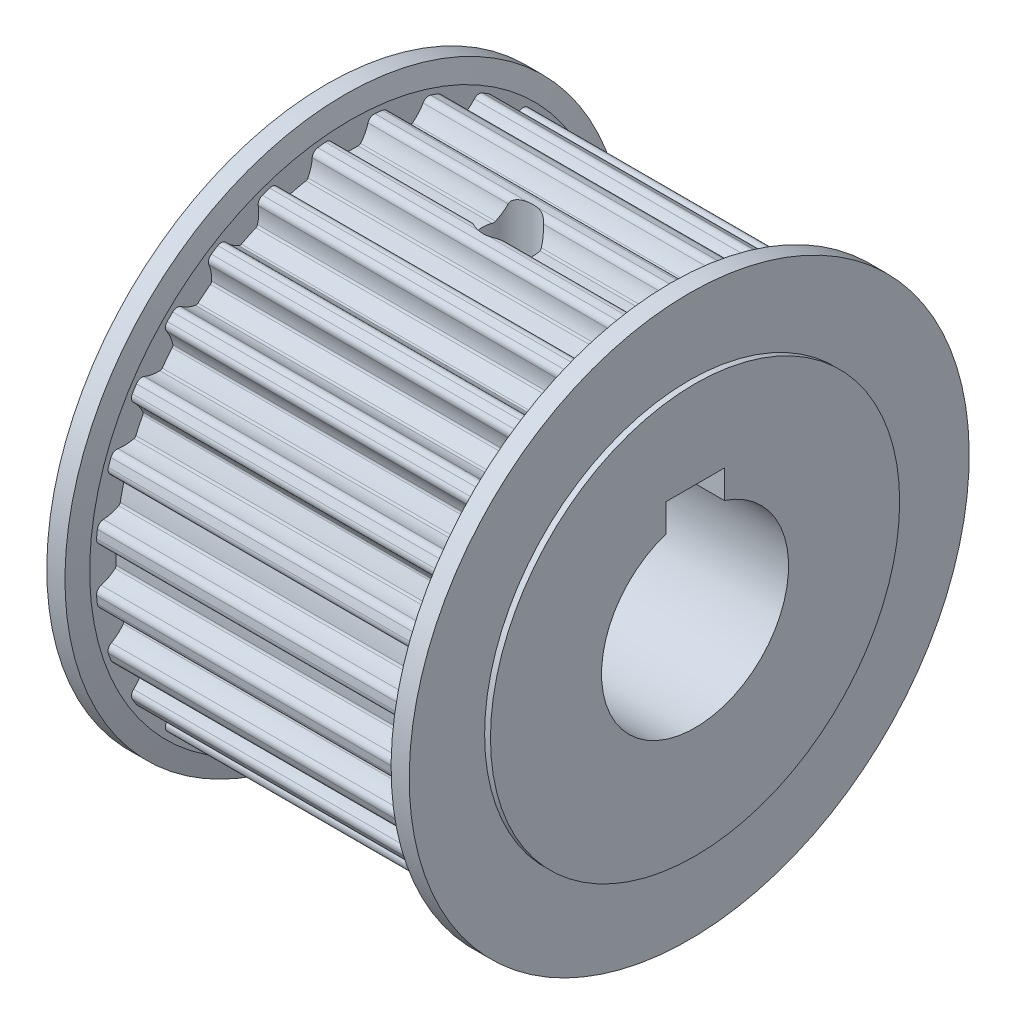
from build123d import *

# Parameters (mm, degrees)
CUT_EXTRUDE1_DEPTH       = 43.67001289
FILLET1_R                = 0.25
FILLET2_R                = 0.55
CIRPATTERN1_COUNT        = 28
FILLET1_OF_CIRPATTERN1_R = 0.25
FILLET2_OF_CIRPATTERN1_R = 0.55
CUT_EXTRUDE4_DEPTH       = 47.596190831
SKETCH24_W               = 2.15
SKETCH24_H               = 21.8
SKETCH25_W               = 2.15
SKETCH25_H               = 21.8


with BuildPart() as part:
    # Sketch1 → Revolve1 (revolve)
    with BuildSketch(Plane.XY, mode=Mode.PRIVATE) as revolve1_sk:
        Polygon((-13.5, 21.8), (-13.5, 17.5), (-16, 17.5), (-16, 0), (16, 0), (16, 17.5), (13.5, 17.5), (13.5, 21.8), align=None)
    revolve(revolve1_sk.sketch.rotate(Axis((16, 0, 0), (-1, 0, 0)), 90), axis=Axis((16, 0, 0), (-1, 0, 0)))

    # Sketch2 → Cut-Extrude1 (cut, through all)
    with BuildSketch(Plane(origin=(13.5, 0, 0), x_dir=(0, 0, -1), z_dir=(1, 0, 0))):
        with BuildLine():
            ThreePointArc((1.625, 21.739350841), (0, 21.8), (-1.625, 21.739350841))
            ThreePointArc((-1.625, 21.739350841), (-1.343515659, 20.815447254), (-0.804781532, 20.013825888))
            ThreePointArc((-0.804781532, 20.013825888), (0, 20.03), (0.804781532, 20.013825888))
            ThreePointArc((0.804781532, 20.013825888), (1.343515659, 20.815447254), (1.625, 21.739350841))
        make_face()
    cut_extrude1 = extrude(amount=-CUT_EXTRUDE1_DEPTH, mode=Mode.SUBTRACT)

    # Fillet1
    fillet1_edges = [part.edges().sort_by_distance(p)[0] for p in [
        (0, 20.013825888, -0.804781532),
        (0, 20.013825888, 0.804781532),
    ]]
    fillet(fillet1_edges, radius=FILLET1_R)

    # Fillet2
    fillet2_edges = [part.edges().sort_by_distance(p)[0] for p in [
        (0, 21.739350841, -1.625),
        (0, 21.739350841, 1.625),
    ]]
    fillet(fillet2_edges, radius=FILLET2_R)

    # CirPattern1: Cut-Extrude1 ×28 about axis
    cirpattern1_axis = Axis((0, 0, 0), (1, 0, 0))
    for i in range(1, CIRPATTERN1_COUNT):
        add(cut_extrude1.rotate(cirpattern1_axis, i * 360 / CIRPATTERN1_COUNT), mode=Mode.SUBTRACT)

    # Fillet1 of CirPattern1
    fillet1_of_cirpattern1_edges = [part.edges().sort_by_distance(p)[0] for p in [
        (0, 19.691118226, 3.66889125),
        (0, 19.33295675, 5.238099208),
        (0, 18.381015673, 7.958590504),
        (0, 17.682652433, 9.408756716),
        (0, 16.149212242, 11.849212799),
        (0, 15.145666086, 13.107619876),
        (0, 13.107619876, 15.145666086),
        (0, 11.849212799, 16.149212242),
        (0, 9.408756716, 17.682652433),
        (0, 7.958590504, 18.381015673),
        (0, 5.238099208, 19.33295675),
        (0, 3.66889125, 19.691118226),
        (0, 0.804781532, 20.013825888),
        (0, -0.804781532, 20.013825888),
        (0, -3.66889125, 19.691118226),
        (0, -5.238099208, 19.33295675),
        (0, -7.958590504, 18.381015673),
        (0, -9.408756716, 17.682652433),
        (0, -11.849212799, 16.149212242),
        (0, -13.107619876, 15.145666086),
        (0, -15.145666086, 13.107619876),
        (0, -16.149212242, 11.849212799),
        (0, -17.682652433, 9.408756716),
        (0, -18.381015673, 7.958590504),
        (0, -19.33295675, 5.238099208),
        (0, -19.691118226, 3.66889125),
        (0, -20.013825888, 0.804781532),
        (0, -20.013825888, -0.804781532),
        (0, -19.691118226, -3.66889125),
        (0, -19.33295675, -5.238099208),
        (0, -18.381015673, -7.958590504),
        (0, -17.682652433, -9.408756716),
        (0, -16.149212242, -11.849212799),
        (0, -15.145666086, -13.107619876),
        (0, -13.107619876, -15.145666086),
        (0, -11.849212799, -16.149212242),
        (0, -9.408756716, -17.682652433),
        (0, -7.958590504, -18.381015673),
        (0, -5.238099208, -19.33295675),
        (0, -3.66889125, -19.691118226),
        (0, -0.804781532, -20.013825888),
        (0, 0.804781532, -20.013825888),
        (0, 3.66889125, -19.691118226),
        (0, 5.238099208, -19.33295675),
        (0, 7.958590504, -18.381015673),
        (0, 9.408756716, -17.682652433),
        (0, 11.849212799, -16.149212242),
        (0, 13.107619876, -15.145666086),
        (0, 15.145666086, -13.107619876),
        (0, 16.149212242, -11.849212799),
        (0, 17.682652433, -9.408756716),
        (0, 18.381015673, -7.958590504),
        (0, 19.33295675, -5.238099208),
        (0, 19.691118226, -3.66889125),
    ]]
    fillet(fillet1_of_cirpattern1_edges, radius=FILLET1_OF_CIRPATTERN1_R)

    # Fillet2 of CirPattern1
    fillet2_of_cirpattern1_edges = [part.edges().sort_by_distance(p)[0] for p in [
        (0, 21.555896446, 3.253202796),
        (0, 20.83270341, 6.42171851),
        (0, 20.291539392, 7.968276419),
        (0, 18.88141724, 10.896425239),
        (0, 18.009679824, 12.28378739),
        (0, 15.983337968, 14.824739708),
        (0, 14.824739708, 15.983337968),
        (0, 12.28378739, 18.009679824),
        (0, 10.896425239, 18.88141724),
        (0, 7.968276419, 20.291539392),
        (0, 6.42171851, 20.83270341),
        (0, 3.253202796, 21.555896446),
        (0, 1.625, 21.739350841),
        (0, -1.625, 21.739350841),
        (0, -3.253202796, 21.555896446),
        (0, -6.42171851, 20.83270341),
        (0, -7.968276419, 20.291539392),
        (0, -10.896425239, 18.88141724),
        (0, -12.28378739, 18.009679824),
        (0, -14.824739708, 15.983337968),
        (0, -15.983337968, 14.824739708),
        (0, -18.009679824, 12.28378739),
        (0, -18.88141724, 10.896425239),
        (0, -20.291539392, 7.968276419),
        (0, -20.83270341, 6.42171851),
        (0, -21.555896446, 3.253202796),
        (0, -21.739350841, 1.625),
        (0, -21.739350841, -1.625),
        (0, -21.555896446, -3.253202796),
        (0, -20.83270341, -6.42171851),
        (0, -20.291539392, -7.968276419),
        (0, -18.88141724, -10.896425239),
        (0, -18.009679824, -12.28378739),
        (0, -15.983337968, -14.824739708),
        (0, -14.824739708, -15.983337968),
        (0, -12.28378739, -18.009679824),
        (0, -10.896425239, -18.88141724),
        (0, -7.968276419, -20.291539392),
        (0, -6.42171851, -20.83270341),
        (0, -3.253202796, -21.555896446),
        (0, -1.625, -21.739350841),
        (0, 1.625, -21.739350841),
        (0, 3.253202796, -21.555896446),
        (0, 6.42171851, -20.83270341),
        (0, 7.968276419, -20.291539392),
        (0, 10.896425239, -18.88141724),
        (0, 12.28378739, -18.009679824),
        (0, 14.824739708, -15.983337968),
        (0, 15.983337968, -14.824739708),
        (0, 18.009679824, -12.28378739),
        (0, 18.88141724, -10.896425239),
        (0, 20.291539392, -7.968276419),
        (0, 20.83270341, -6.42171851),
        (0, 21.555896446, -3.253202796),
    ]]
    fillet(fillet2_of_cirpattern1_edges, radius=FILLET2_OF_CIRPATTERN1_R)

    # Sketch3 → Revolve3 (revolve)
    with BuildSketch(Plane.XY):
        Polygon((-15.5, 23.95), (-15.5, 17.5), (-13.5, 17.5), (-13.5, 22.28), (-13.947475151, 23.95), align=None)
        Polygon((15.5, 23.95), (15.5, 17.5), (13.5, 17.5), (13.5, 22.28), (13.947475151, 23.95), align=None)
    revolve(axis=Axis((16, 0, 0), (-1, 0, 0)))

    # Sketch8 → Cut-Extrude4 (cut, through all)
    with BuildSketch(Plane.ZY.offset(16)):
        with BuildLine():
            Line((-2.5, 7.599342077), (-2.5, 10))
            Line((-2.5, 10), (2.5, 10))
            Line((2.5, 10), (2.5, 7.599342077))
            ThreePointArc((2.5, 7.599342077), (0, -8), (-2.5, 7.599342077))
        make_face()
    extrude(amount=-CUT_EXTRUDE4_DEPTH, mode=Mode.SUBTRACT)

    # Sketch24 → Cut-Revolve8 (revolve, cut)
    with BuildSketch(Plane.XY, mode=Mode.PRIVATE) as cut_revolve8_sk:
        with Locations((1.075, 10.9)):
            Rectangle(SKETCH24_W, SKETCH24_H)
    revolve(cut_revolve8_sk.sketch.rotate(Axis((0, 0, 0), (0, 1, 0)), 341.369076374), axis=Axis((0, 0, 0), (0, 1, 0)), mode=Mode.SUBTRACT)

    # Sketch25 → Cut-Revolve9 (revolve, cut)
    with BuildSketch(Plane(origin=(0, 0, 0), x_dir=(1, 0, 0), z_dir=(0, 0.8660254037844364, -0.5000000000000041)), mode=Mode.PRIVATE) as cut_revolve9_sk:
        with Locations((-1.075, 10.9)):
            Rectangle(SKETCH25_W, SKETCH25_H)
    revolve(cut_revolve9_sk.sketch.rotate(Axis((0, 0, 0), (0, -0.5000000000000041, -0.8660254037844364)), 270), axis=Axis((0, 0, 0), (0, -0.5000000000000041, -0.8660254037844364)), mode=Mode.SUBTRACT)


solid = part.part
